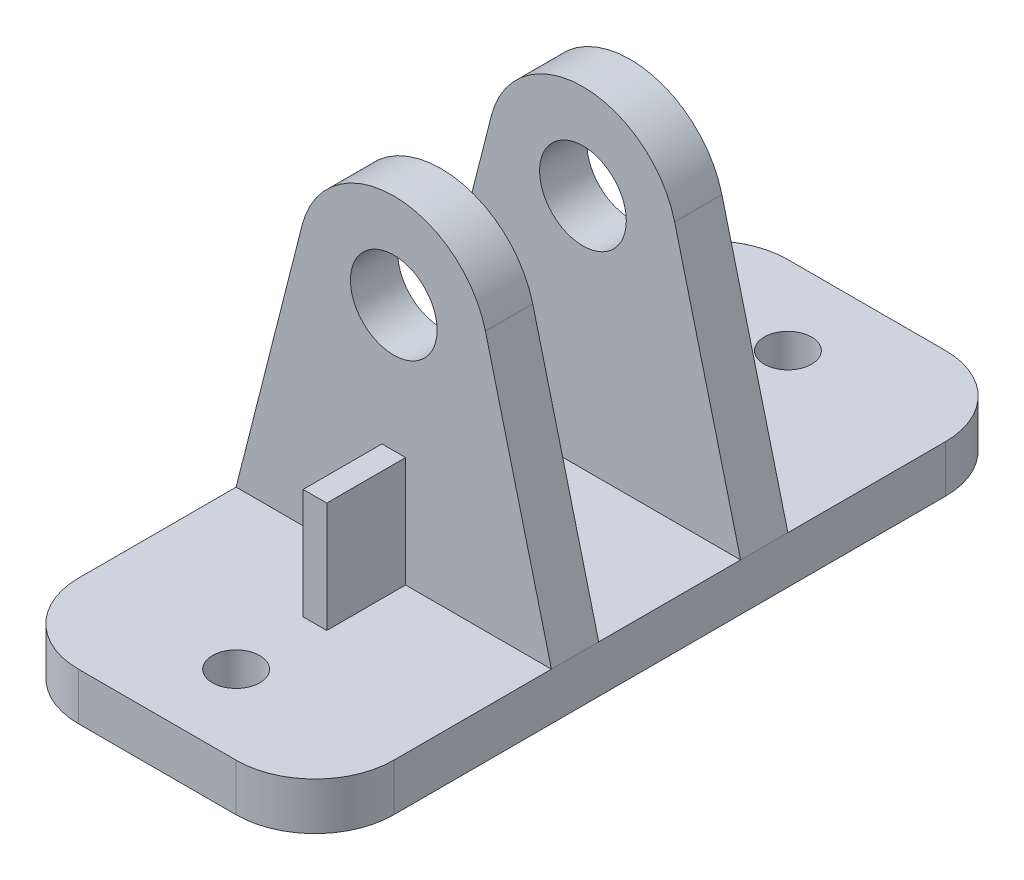
SolidWorks part; units mm, degrees
ref_plane "Front Plane" through (0, 0, 0) normal (0, 0, 1) x (1, 0, 0)
ref_plane "Top Plane" through (0, 0, 0) normal (0, 1, 0) x (1, 0, 0)
ref_plane "Right Plane" through (0, 0, 0) normal (1, 0, 0) x (0, 0, -1)
sketch "Sketch 1" plane through (0, 0, 0) normal (0, 1, 0) x (1, 0, 0)
  line L1 (-100, -75) -> (100, -75)
  line L2 (-100, -75) -> (-100, 75)
  line L3 (-100, 75) -> (100, 75)
  line L4 (100, -75) -> (100, 75)
  line L5 (-100, -75) -> (100, 75) construction
  line L6 (-100, 75) -> (100, -75) construction
  point P0 (0, 0)
  dimension "D1" = 200
  dimension "D2" = 150
extrude "Boss-Extrude 1" add sketch "Sketch 1" along normal blind 30
sketch "Sketch 2" plane through (0, 0, 75) normal (0, 0, 1) x (1, 0, 0)
  line L0 (0, -7.9075) -> (0, 168.2922) construction
  line L1 (-100, 0) -> (100, 0) construction
  line L2 (-58.1538, 194.7692) -> (-100, 30)
  line L3 (-100, 30) -> (100, 30) construction
  line L4 (-100, 30) -> (-100, 0) construction
  line L5 (-100, 30) -> (100, 30)
  line L6 (58.1538, 194.7692) -> (100, 30)
  circle A0 centre (0, 180) radius 27.5
  arc A1 (58.1538, 194.7692) -> (-58.1538, 194.7692) centre (0, 180) ccw
  point P17 (0, 30)
  dimension "D1" = 55
  dimension "D2" = 180
  dimension "D3" = 60
extrude "Boss-Extrude 2" add sketch "Sketch 2" against normal blind 30
sketch "Sketch 4" plane through (0, 0, 75) normal (0, 0, 1) x (1, 0, 0)
  line L0 (0, -12.2336) -> (0, 150.8827) construction
  line L1 (-100, 0) -> (100, 0) construction
  line L2 (-7.5, 100) -> (7.5, 100)
  line L3 (-7.5, 100) -> (-7.5, 0)
  line L4 (-7.5, 0) -> (7.5, 0)
  line L5 (7.5, 100) -> (7.5, 0)
  line L6 (-7.5, 100) -> (7.5, 0) construction
  line L7 (-7.5, 0) -> (7.5, 100) construction
  point P3 (0, 50)
  dimension "D1" = 100
  dimension "15" = 15
extrude "Boss-Extrude 3" add sketch "Sketch 4" along normal blind 50
mirror "Mirror 1" about plane through (0, 0, 0) normal (0, 0, 1) of "Boss-Extrude 2", "Boss-Extrude 3"
sketch "Sketch 5" plane through (0, 0, 0) normal (0, -1, 0) x (1, 0, 0)
  line L0 (-100, -75) -> (-100, 75) construction
  line L1 (100, -225) -> (-100, -225)
  line L2 (100, -225) -> (100, 225)
  line L3 (100, 225) -> (-100, 225)
  line L4 (-100, -225) -> (-100, 225)
  line L5 (100, -225) -> (-100, 225) construction
  line L6 (100, 225) -> (-100, -225) construction
  line L7 (0, -312.6276) -> (0, 307.996) construction
  line L8 (-7.5, -75) -> (-100, -75) construction
  line L9 (-125.9194, -175) -> (134.6035, -175) construction
  line L10 (-7.5, -125) -> (7.5, -125) construction
  line L11 (-132.1053, 0) -> (125.2238, 0) construction
  circle A0 centre (0, -175) radius 15
  circle A1 centre (0, 175) radius 15
  point P0 (0, 0)
  dimension "D2" = 30
  dimension "D1" = 150
extrude "Boss-Extrude 4" add sketch "Sketch 5" against normal up to surface (30 mm away) up to face at (0, 30, 0)
fillet "Fillet 1" radius 50 4 edges at (100, 15, 225) (-100, 15, 225) (100, 15, -225) (-100, 15, -225)
